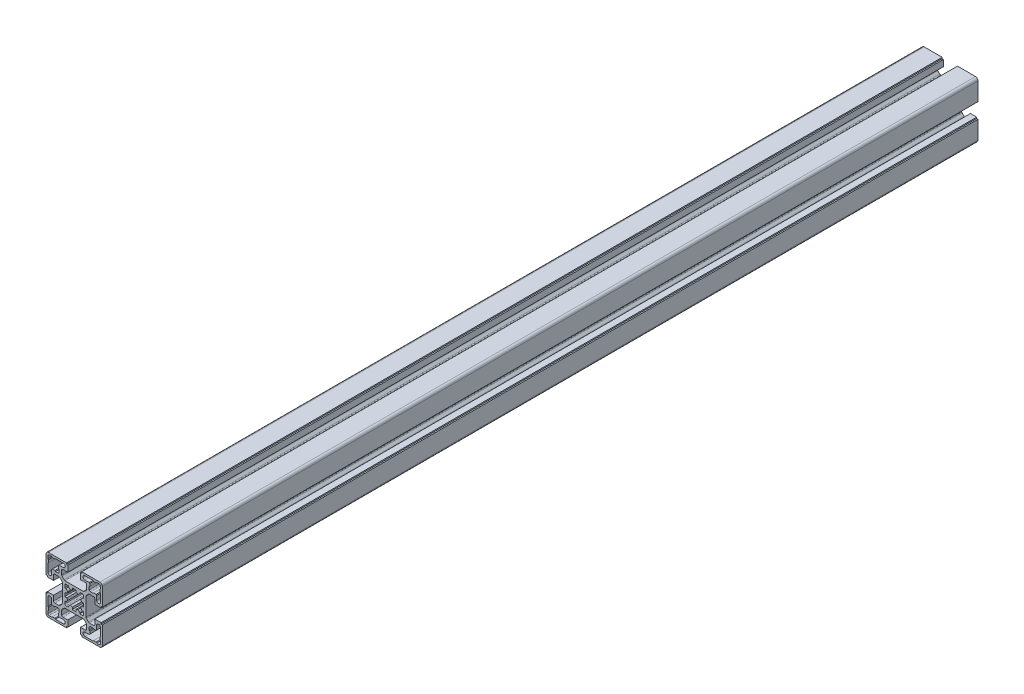
from build123d import *

# Parameters (mm, degrees)
EXTRUDE_1_DEPTH = 700


with BuildPart() as part:
    # 草图1 → 拉伸1 (new body)
    with BuildSketch(Plane.XY):
        with BuildLine():
            Line((33.706586033, 40.501982097), (35.388566549, 38.820001582))
            ThreePointArc((35.388566549, 38.820001582), (35.712989897, 38.603228831), (36.09567333, 38.527108363))
            Line((36.09567333, 38.527108363), (39.413692815, 38.527108363))
            ThreePointArc((39.413692815, 38.527108363), (40.120799596, 38.820001582), (40.413692815, 39.527108363))
            Line((40.413692815, 39.527108363), (40.413692815, 43.427108363))
            Line((40.413692815, 43.427108363), (45.413692815, 43.427108363))
            Line((45.413692815, 43.427108363), (45.413692815, 42.427108363))
            Line((45.413692815, 42.427108363), (46.413692815, 42.427108363))
            Line((46.413692815, 42.427108363), (46.413692815, 28.027108363))
            ThreePointArc((46.413692815, 28.027108363), (45.827906377, 26.612894801), (44.413692815, 26.027108363))
            Line((44.413692815, 26.027108363), (30.013692814, 26.027108363))
            Line((30.013692814, 26.027108363), (30.013692814, 27.027108363))
            Line((30.013692814, 27.027108363), (29.013692814, 27.027108363))
            Line((29.013692814, 27.027108363), (29.013692814, 32.027108363))
            Line((29.013692814, 32.027108363), (32.913692814, 32.027108363))
            ThreePointArc((32.913692814, 32.027108363), (33.620799596, 32.320001582), (33.913692814, 33.027108363))
            Line((33.913692814, 33.027108363), (33.913692814, 36.345127848))
            ThreePointArc((33.913692814, 36.345127848), (33.837572347, 36.72781128), (33.620799596, 37.052234629))
            Line((33.620799596, 37.052234629), (31.938819081, 38.734215144))
            ThreePointArc((31.938819081, 38.734215144), (31.614395732, 38.950987895), (31.231712299, 39.027108363))
            Line((31.231712299, 39.027108363), (16.59567333, 39.027108363))
            ThreePointArc((16.59567333, 39.027108363), (16.212989897, 38.950987895), (15.888566548, 38.734215144))
            Line((15.888566548, 38.734215144), (14.206586033, 37.052234629))
            ThreePointArc((14.206586033, 37.052234629), (13.989813282, 36.72781128), (13.913692814, 36.345127848))
            Line((13.913692814, 36.345127848), (13.913692814, 33.027108363))
            ThreePointArc((13.913692814, 33.027108363), (14.206586033, 32.320001582), (14.913692814, 32.027108363))
            Line((14.913692814, 32.027108363), (18.813692815, 32.027108363))
            Line((18.813692815, 32.027108363), (18.813692815, 27.027108363))
            Line((18.813692815, 27.027108363), (17.813692815, 27.027108363))
            Line((17.813692815, 27.027108363), (17.813692815, 26.027108363))
            Line((17.813692815, 26.027108363), (3.413692814, 26.027108363))
            ThreePointArc((3.413692814, 26.027108363), (1.999479252, 26.612894801), (1.413692814, 28.027108363))
            Line((1.413692814, 28.027108363), (1.413692814, 42.427108363))
            Line((1.413692814, 42.427108363), (2.413692814, 42.427108363))
            Line((2.413692814, 42.427108363), (2.413692814, 43.427108363))
            Line((2.413692814, 43.427108363), (7.413692814, 43.427108363))
            Line((7.413692814, 43.427108363), (7.413692814, 39.527108363))
            ThreePointArc((7.413692814, 39.527108363), (7.706586033, 38.820001582), (8.413692814, 38.527108363))
            Line((8.413692814, 38.527108363), (11.731712299, 38.527108363))
            ThreePointArc((11.731712299, 38.527108363), (12.114395732, 38.603228831), (12.43881908, 38.820001582))
            Line((12.43881908, 38.820001582), (14.120799595, 40.501982097))
            ThreePointArc((14.120799595, 40.501982097), (14.337572347, 40.826405446), (14.413692814, 41.209088878))
            Line((14.413692814, 41.209088878), (14.413692814, 55.845127848))
            ThreePointArc((14.413692814, 55.845127848), (14.337572347, 56.22781128), (14.120799595, 56.552234629))
            Line((14.120799595, 56.552234629), (12.43881908, 58.234215144))
            ThreePointArc((12.43881908, 58.234215144), (12.114395732, 58.450987896), (11.731712299, 58.527108363))
            Line((11.731712299, 58.527108363), (8.413692814, 58.527108363))
            ThreePointArc((8.413692814, 58.527108363), (7.706586033, 58.234215144), (7.413692814, 57.527108363))
            Line((7.413692814, 57.527108363), (7.413692814, 53.627108363))
            Line((7.413692814, 53.627108363), (2.413692814, 53.627108363))
            Line((2.413692814, 53.627108363), (2.413692814, 54.627108363))
            Line((2.413692814, 54.627108363), (1.413692814, 54.627108363))
            Line((1.413692814, 54.627108363), (1.413692814, 69.027108363))
            ThreePointArc((1.413692814, 69.027108363), (1.999479252, 70.441321926), (3.413692814, 71.027108363))
            Line((3.413692814, 71.027108363), (17.813692815, 71.027108363))
            Line((17.813692815, 71.027108363), (17.813692815, 70.027108363))
            Line((17.813692815, 70.027108363), (18.813692815, 70.027108363))
            Line((18.813692815, 70.027108363), (18.813692815, 65.027108363))
            Line((18.813692815, 65.027108363), (14.913692814, 65.027108363))
            ThreePointArc((14.913692814, 65.027108363), (14.206586033, 64.734215145), (13.913692814, 64.027108363))
            Line((13.913692814, 64.027108363), (13.913692814, 60.709088878))
            ThreePointArc((13.913692814, 60.709088878), (13.989813282, 60.326405446), (14.206586033, 60.001982097))
            Line((14.206586033, 60.001982097), (15.888566548, 58.320001582))
            ThreePointArc((15.888566548, 58.320001582), (16.212989897, 58.103228831), (16.59567333, 58.027108363))
            Line((16.59567333, 58.027108363), (31.231712299, 58.027108363))
            ThreePointArc((31.231712299, 58.027108363), (31.614395732, 58.103228831), (31.938819081, 58.320001582))
            Line((31.938819081, 58.320001582), (33.620799596, 60.001982097))
            ThreePointArc((33.620799596, 60.001982097), (33.837572347, 60.326405446), (33.913692814, 60.709088878))
            Line((33.913692814, 60.709088878), (33.913692814, 64.027108363))
            ThreePointArc((33.913692814, 64.027108363), (33.620799596, 64.734215145), (32.913692814, 65.027108363))
            Line((32.913692814, 65.027108363), (29.013692814, 65.027108363))
            Line((29.013692814, 65.027108363), (29.013692814, 70.027108363))
            Line((29.013692814, 70.027108363), (30.013692814, 70.027108363))
            Line((30.013692814, 70.027108363), (30.013692814, 71.027108363))
            Line((30.013692814, 71.027108363), (44.413692815, 71.027108363))
            ThreePointArc((44.413692815, 71.027108363), (45.827906377, 70.441321926), (46.413692815, 69.027108363))
            Line((46.413692815, 69.027108363), (46.413692815, 54.627108363))
            Line((46.413692815, 54.627108363), (45.413692815, 54.627108363))
            Line((45.413692815, 54.627108363), (45.413692815, 53.627108363))
            Line((45.413692815, 53.627108363), (40.413692815, 53.627108363))
            Line((40.413692815, 53.627108363), (40.413692815, 57.527108363))
            ThreePointArc((40.413692815, 57.527108363), (40.120799596, 58.234215144), (39.413692815, 58.527108363))
            Line((39.413692815, 58.527108363), (36.09567333, 58.527108363))
            ThreePointArc((36.09567333, 58.527108363), (35.712989897, 58.450987896), (35.388566549, 58.234215144))
            Line((35.388566549, 58.234215144), (33.706586033, 56.552234629))
            ThreePointArc((33.706586033, 56.552234629), (33.489813282, 56.22781128), (33.413692815, 55.845127848))
            Line((33.413692815, 55.845127848), (33.413692815, 41.209088878))
            ThreePointArc((33.413692815, 41.209088878), (33.489813282, 40.826405446), (33.706586033, 40.501982097))
        make_face()
        with BuildLine():
            Line((30.535013158, 44.027108363), (29.082272168, 45.479849354))
            ThreePointArc((29.082272168, 45.479849354), (29.45697001, 46.231007769), (29.723167834, 47.027108363))
            Line((29.723167834, 47.027108363), (31.413692814, 47.027108363))
            Line((31.413692814, 47.027108363), (31.413692814, 50.027108363))
            Line((31.413692814, 50.027108363), (29.723167834, 50.027108363))
            ThreePointArc((29.723167834, 50.027108363), (29.45697001, 50.823208957), (29.082272168, 51.574367373))
            Line((29.082272168, 51.574367373), (30.535013158, 53.027108363))
            Line((30.535013158, 53.027108363), (31.413692814, 53.027108363))
            Line((31.413692814, 53.027108363), (31.413692814, 55.027108363))
            ThreePointArc((31.413692814, 55.027108363), (31.120799596, 55.734215144), (30.413692814, 56.027108363))
            Line((30.413692814, 56.027108363), (28.413692814, 56.027108363))
            Line((28.413692814, 56.027108363), (28.413692814, 55.148428707))
            Line((28.413692814, 55.148428707), (26.960951824, 53.695687716))
            ThreePointArc((26.960951824, 53.695687716), (26.209793409, 54.070385558), (25.413692814, 54.336583382))
            Line((25.413692814, 54.336583382), (25.413692814, 56.027108363))
            Line((25.413692814, 56.027108363), (22.413692814, 56.027108363))
            Line((22.413692814, 56.027108363), (22.413692814, 54.336583382))
            ThreePointArc((22.413692814, 54.336583382), (21.61759222, 54.070385558), (20.866433805, 53.695687716))
            Line((20.866433805, 53.695687716), (19.413692814, 55.148428707))
            Line((19.413692814, 55.148428707), (19.413692814, 56.027108363))
            Line((19.413692814, 56.027108363), (17.413692814, 56.027108363))
            ThreePointArc((17.413692814, 56.027108363), (16.706586033, 55.734215144), (16.413692814, 55.027108363))
            Line((16.413692814, 55.027108363), (16.413692814, 53.027108363))
            Line((16.413692814, 53.027108363), (17.292372471, 53.027108363))
            Line((17.292372471, 53.027108363), (18.745113461, 51.574367373))
            ThreePointArc((18.745113461, 51.574367373), (18.370415619, 50.823208957), (18.104217795, 50.027108363))
            Line((18.104217795, 50.027108363), (16.413692814, 50.027108363))
            Line((16.413692814, 50.027108363), (16.413692814, 47.027108363))
            Line((16.413692814, 47.027108363), (18.104217795, 47.027108363))
            ThreePointArc((18.104217795, 47.027108363), (18.370415619, 46.231007769), (18.745113461, 45.479849354))
            Line((18.745113461, 45.479849354), (17.292372471, 44.027108363))
            Line((17.292372471, 44.027108363), (16.413692814, 44.027108363))
            Line((16.413692814, 44.027108363), (16.413692814, 42.027108363))
            ThreePointArc((16.413692814, 42.027108363), (16.706586033, 41.320001582), (17.413692814, 41.027108363))
            Line((17.413692814, 41.027108363), (19.413692814, 41.027108363))
            Line((19.413692814, 41.027108363), (19.413692814, 41.90578802))
            Line((19.413692814, 41.90578802), (20.866433805, 43.35852901))
            ThreePointArc((20.866433805, 43.35852901), (21.61759222, 42.983831168), (22.413692814, 42.717633344))
            Line((22.413692814, 42.717633344), (22.413692814, 41.027108363))
            Line((22.413692814, 41.027108363), (25.413692814, 41.027108363))
            Line((25.413692814, 41.027108363), (25.413692814, 42.717633344))
            ThreePointArc((25.413692814, 42.717633344), (26.209793409, 42.983831168), (26.960951824, 43.35852901))
            Line((26.960951824, 43.35852901), (28.413692814, 41.90578802))
            Line((28.413692814, 41.90578802), (28.413692814, 41.027108363))
            Line((28.413692814, 41.027108363), (30.413692814, 41.027108363))
            ThreePointArc((30.413692814, 41.027108363), (31.120799596, 41.320001582), (31.413692814, 42.027108363))
            Line((31.413692814, 42.027108363), (31.413692814, 44.027108363))
            Line((31.413692814, 44.027108363), (30.535013158, 44.027108363))
        make_face(mode=Mode.SUBTRACT)
        with BuildLine():
            Line((11.413692814, 66.027108363), (11.913692814, 66.527108364))
            Line((11.913692814, 66.527108364), (15.313692814, 66.527108364))
            ThreePointArc((15.313692814, 66.527108364), (16.813692814, 68.027108363), (15.313692814, 69.527108363))
            Line((15.313692814, 69.527108363), (8.913692815, 69.527108363))
            Line((8.913692815, 69.527108363), (8.413692814, 69.027108363))
            Line((8.413692814, 69.027108363), (6.413692814, 69.027108363))
            Line((6.413692814, 69.027108363), (5.913692814, 69.527108363))
            Line((5.913692814, 69.527108363), (3.913692814, 69.527108363))
            ThreePointArc((3.913692814, 69.527108363), (3.206586033, 69.234215145), (2.913692814, 68.527108363))
            Line((2.913692814, 68.527108363), (2.913692814, 66.527108363))
            Line((2.913692814, 66.527108363), (3.413692814, 66.027108363))
            Line((3.413692814, 66.027108363), (3.413692814, 64.027108363))
            Line((3.413692814, 64.027108363), (2.913692814, 63.527108363))
            Line((2.913692814, 63.527108363), (2.913692814, 57.127108364))
            ThreePointArc((2.913692814, 57.127108364), (4.413692814, 55.627108364), (5.913692814, 57.127108364))
            Line((5.913692814, 57.127108364), (5.913692814, 60.527108363))
            Line((5.913692814, 60.527108363), (6.413692814, 61.027108363))
            Line((6.413692814, 61.027108363), (8.413692814, 61.027108363))
            Line((8.413692814, 61.027108363), (8.913692814, 60.527108363))
            Line((8.913692814, 60.527108363), (10.913692814, 60.527108363))
            ThreePointArc((10.913692814, 60.527108363), (11.620799595, 60.820001582), (11.913692814, 61.527108363))
            Line((11.913692814, 61.527108363), (11.913692814, 63.527108363))
            Line((11.913692814, 63.527108363), (11.413692814, 64.027108363))
            Line((11.413692814, 64.027108363), (11.413692814, 66.027108363))
        make_face(mode=Mode.SUBTRACT)
        with BuildLine():
            Line((11.913692815, 30.527108363), (11.413692814, 31.027108363))
            Line((11.413692814, 31.027108363), (11.413692814, 33.027108363))
            Line((11.413692814, 33.027108363), (11.913692815, 33.527108363))
            Line((11.913692815, 33.527108363), (11.913692815, 35.527108363))
            ThreePointArc((11.913692815, 35.527108363), (11.620799596, 36.234215144), (10.913692815, 36.527108363))
            Line((10.913692815, 36.527108363), (8.913692815, 36.527108363))
            Line((8.913692815, 36.527108363), (8.413692815, 36.027108363))
            Line((8.413692815, 36.027108363), (6.413692814, 36.027108363))
            Line((6.413692814, 36.027108363), (5.913692814, 36.527108363))
            Line((5.913692814, 36.527108363), (5.913692814, 39.927108363))
            ThreePointArc((5.913692814, 39.927108363), (4.413692814, 41.427108363), (2.913692814, 39.927108363))
            Line((2.913692814, 39.927108363), (2.913692814, 33.527108363))
            Line((2.913692814, 33.527108363), (3.413692814, 33.027108363))
            Line((3.413692814, 33.027108363), (3.413692814, 31.027108363))
            Line((3.413692814, 31.027108363), (2.913692814, 30.527108363))
            Line((2.913692814, 30.527108363), (2.913692814, 28.527108363))
            ThreePointArc((2.913692814, 28.527108363), (3.206586033, 27.820001582), (3.913692814, 27.527108363))
            Line((3.913692814, 27.527108363), (5.913692814, 27.527108363))
            Line((5.913692814, 27.527108363), (6.413692814, 28.027108363))
            Line((6.413692814, 28.027108363), (8.413692814, 28.027108363))
            Line((8.413692814, 28.027108363), (8.913692815, 27.527108363))
            Line((8.913692815, 27.527108363), (15.313692814, 27.527108363))
            ThreePointArc((15.313692814, 27.527108363), (16.813692814, 29.027108363), (15.313692814, 30.527108363))
            Line((15.313692814, 30.527108363), (11.913692815, 30.527108363))
        make_face(mode=Mode.SUBTRACT)
        with BuildLine():
            Line((41.913692815, 36.527108363), (41.413692815, 36.027108363))
            Line((41.413692815, 36.027108363), (39.413692815, 36.027108363))
            Line((39.413692815, 36.027108363), (38.913692814, 36.527108363))
            Line((38.913692814, 36.527108363), (36.913692815, 36.527108363))
            ThreePointArc((36.913692815, 36.527108363), (36.206586033, 36.234215145), (35.913692815, 35.527108363))
            Line((35.913692815, 35.527108363), (35.913692815, 33.527108364))
            Line((35.913692815, 33.527108364), (36.413692815, 33.027108363))
            Line((36.413692815, 33.027108363), (36.413692815, 31.027108363))
            Line((36.413692815, 31.027108363), (35.913692815, 30.527108363))
            Line((35.913692815, 30.527108363), (32.513692815, 30.527108363))
            ThreePointArc((32.513692815, 30.527108363), (31.013692815, 29.027108363), (32.513692815, 27.527108363))
            Line((32.513692815, 27.527108363), (38.913692814, 27.527108363))
            Line((38.913692814, 27.527108363), (39.413692814, 28.027108363))
            Line((39.413692814, 28.027108363), (41.413692814, 28.027108363))
            Line((41.413692814, 28.027108363), (41.913692815, 27.527108363))
            Line((41.913692815, 27.527108363), (43.913692815, 27.527108363))
            ThreePointArc((43.913692815, 27.527108363), (44.620799596, 27.820001582), (44.913692815, 28.527108363))
            Line((44.913692815, 28.527108363), (44.913692815, 30.527108363))
            Line((44.913692815, 30.527108363), (44.413692814, 31.027108363))
            Line((44.413692814, 31.027108363), (44.413692814, 33.027108363))
            Line((44.413692814, 33.027108363), (44.913692815, 33.527108364))
            Line((44.913692815, 33.527108364), (44.913692815, 39.927108363))
            ThreePointArc((44.913692815, 39.927108363), (43.413692815, 41.427108363), (41.913692815, 39.927108363))
            Line((41.913692815, 39.927108363), (41.913692815, 36.527108363))
        make_face(mode=Mode.SUBTRACT)
        with BuildLine():
            Line((35.913692815, 66.527108363), (36.413692815, 66.027108363))
            Line((36.413692815, 66.027108363), (36.413692815, 64.027108363))
            Line((36.413692815, 64.027108363), (35.913692815, 63.527108363))
            Line((35.913692815, 63.527108363), (35.913692815, 61.527108363))
            ThreePointArc((35.913692815, 61.527108363), (36.206586033, 60.820001582), (36.913692815, 60.527108363))
            Line((36.913692815, 60.527108363), (38.913692814, 60.527108363))
            Line((38.913692814, 60.527108363), (39.413692815, 61.027108364))
            Line((39.413692815, 61.027108364), (41.413692815, 61.027108364))
            Line((41.413692815, 61.027108364), (41.913692815, 60.527108363))
            Line((41.913692815, 60.527108363), (41.913692815, 57.127108364))
            ThreePointArc((41.913692815, 57.127108364), (43.413692815, 55.627108364), (44.913692815, 57.127108364))
            Line((44.913692815, 57.127108364), (44.913692815, 63.527108363))
            Line((44.913692815, 63.527108363), (44.413692815, 64.027108363))
            Line((44.413692815, 64.027108363), (44.413692815, 66.027108363))
            Line((44.413692815, 66.027108363), (44.913692815, 66.527108363))
            Line((44.913692815, 66.527108363), (44.913692815, 68.527108363))
            ThreePointArc((44.913692815, 68.527108363), (44.620799596, 69.234215145), (43.913692815, 69.527108363))
            Line((43.913692815, 69.527108363), (41.913692815, 69.527108363))
            Line((41.913692815, 69.527108363), (41.413692814, 69.027108363))
            Line((41.413692814, 69.027108363), (39.413692814, 69.027108363))
            Line((39.413692814, 69.027108363), (38.913692814, 69.527108363))
            Line((38.913692814, 69.527108363), (32.513692815, 69.527108363))
            ThreePointArc((32.513692815, 69.527108363), (31.013692815, 68.027108363), (32.513692815, 66.527108363))
            Line((32.513692815, 66.527108363), (35.913692815, 66.527108363))
        make_face(mode=Mode.SUBTRACT)
    extrude(amount=EXTRUDE_1_DEPTH)


solid = part.part
